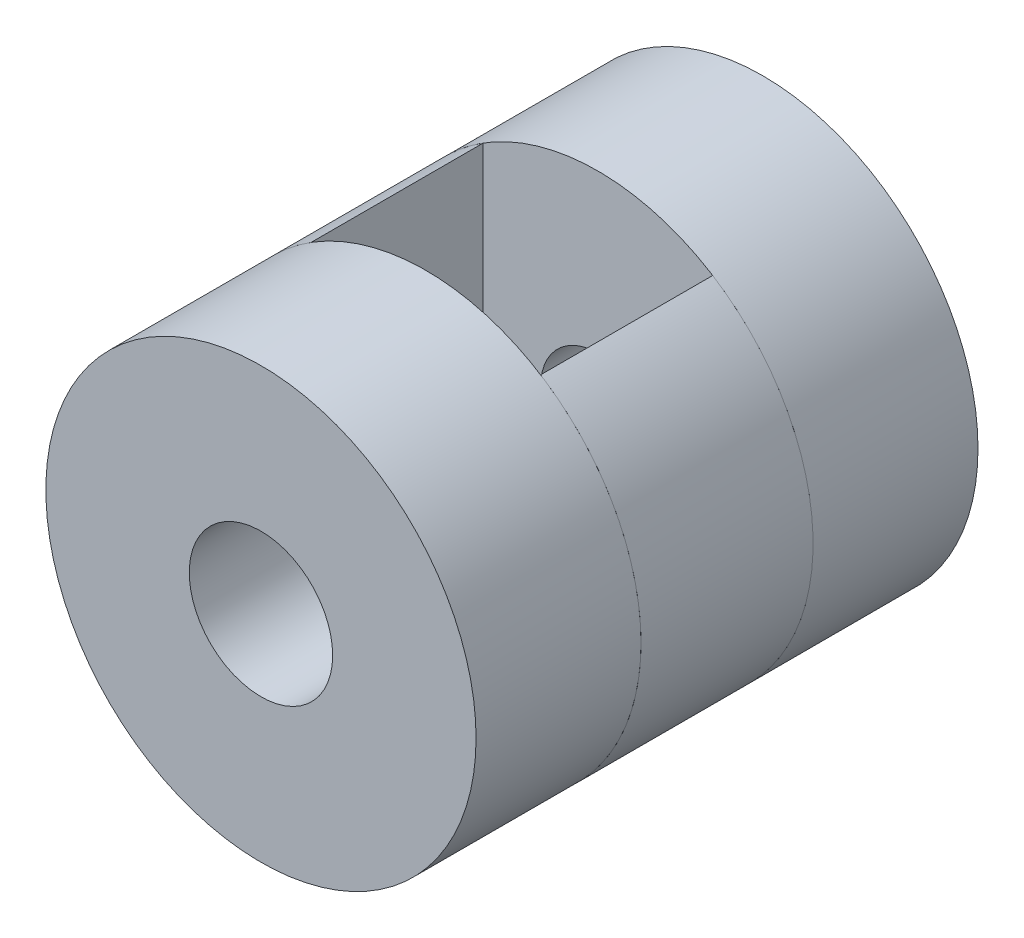
from build123d import *

# Parameters (mm, degrees)
SKETCH1_R              = 15
SKETCH1_R_2            = 4
BOSS_EXTRUDE1_DEPTH    = 17.5
SKETCH2_W              = 16
SKETCH2_H              = 12
CUT_EXTRUDE1_DEPTH     = 17.5
CUT_EXTRUDE2_REACH     = 42.927
SKETCH3_R              = 5
SPLIT1_SURFACE_1_BACK  = 56
SPLIT1_SURFACE_1_DEPTH = 112
SPLIT1_SURFACE_2_BACK  = 56
SPLIT1_SURFACE_2_DEPTH = 112


with BuildPart() as part:
    # Sketch1 → Boss-Extrude1 (new, symmetric)
    with BuildSketch(Plane.XY):
        Circle(SKETCH1_R)
        Circle(SKETCH1_R_2, mode=Mode.SUBTRACT)
    extrude(amount=BOSS_EXTRUDE1_DEPTH, both=True)

    # Sketch2 → Cut-Extrude1 (cut, symmetric)
    with BuildSketch(Plane(origin=(0, 0, 0), x_dir=(1, 0, 0), z_dir=(0, 1, 0))):
        Rectangle(SKETCH2_W, SKETCH2_H)
    extrude(amount=CUT_EXTRUDE1_DEPTH, both=True, mode=Mode.SUBTRACT)

    # Sketch3 → Cut-Extrude2 (cut, up to next)
    with BuildSketch(Plane.XY.offset(17.5), mode=Mode.PRIVATE) as cut_extrude2_sk1:
        Circle(SKETCH3_R)
    cut_extrude2_tool1 = extrude(cut_extrude2_sk1.sketch, amount=-CUT_EXTRUDE2_REACH, mode=Mode.PRIVATE) & part.part
    add(cut_extrude2_tool1.solids().sort_by_distance((0, 0, 17.5))[0], mode=Mode.SUBTRACT)


with BuildPart() as body_2:
    # Split1: the piece behind the surface
    add(part.part)
    # Split1 surface: a surface, the sketch's curves swept straight by 112 mm
    with BuildLine(Plane(origin=(0, 0, 0), x_dir=(1, 0, 0), z_dir=(0, 1, 0)).offset(-SPLIT1_SURFACE_1_BACK), mode=Mode.PRIVATE) as split1_surface_1_path:
        Line((-15, 6), (15, 6))
        Line((15, 6), (15, -6))
        Line((15, -6), (-15, -6))
        Line((-15, -6), (-15, 6))
    split1_surface_1 = Shell.extrude(split1_surface_1_path.wire(), (0 * SPLIT1_SURFACE_1_DEPTH, 1 * SPLIT1_SURFACE_1_DEPTH, 0 * SPLIT1_SURFACE_1_DEPTH))
    split(bisect_by=split1_surface_1, keep=Keep.BOTTOM)


with BuildPart() as part_1:
    add(part.part)

    # Split1: split by a surface, the side it looks to stays
    # Split1 surface: a surface, the sketch's curves swept straight by 112 mm
    with BuildLine(Plane(origin=(0, 0, 0), x_dir=(1, 0, 0), z_dir=(0, 1, 0)).offset(-SPLIT1_SURFACE_2_BACK), mode=Mode.PRIVATE) as split1_surface_2_path:
        Line((-15, 6), (15, 6))
        Line((15, 6), (15, -6))
        Line((15, -6), (-15, -6))
        Line((-15, -6), (-15, 6))
    split1_surface_2 = Shell.extrude(split1_surface_2_path.wire(), (0 * SPLIT1_SURFACE_2_DEPTH, 1 * SPLIT1_SURFACE_2_DEPTH, 0 * SPLIT1_SURFACE_2_DEPTH))
    split(bisect_by=split1_surface_2, keep=Keep.TOP)


solid = Compound([body_2.part, part_1.part])
